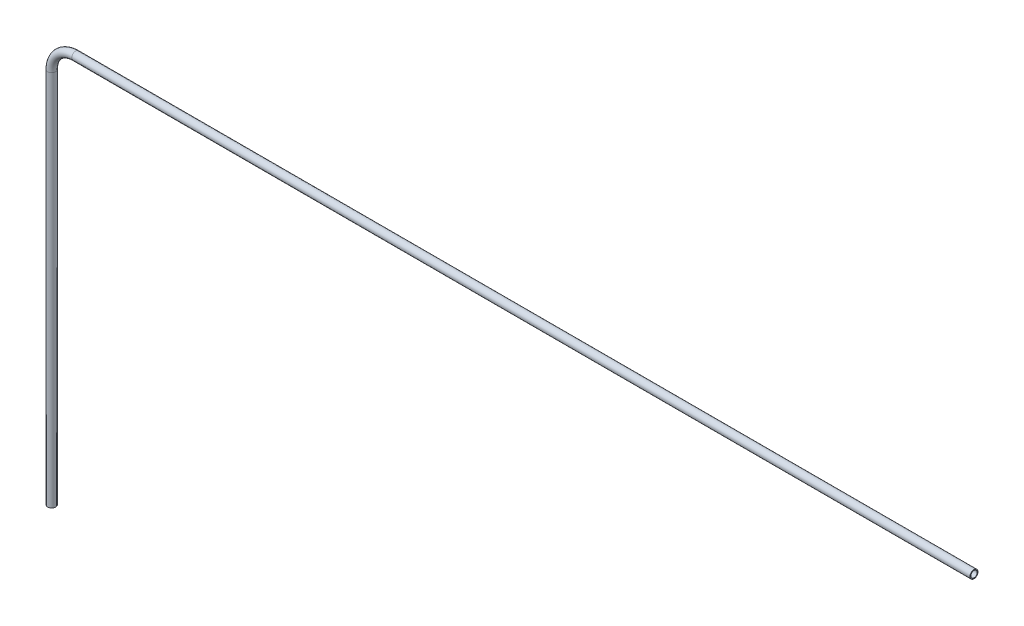
from build123d import *

# Parameters (mm, degrees)
SWEEP_THIN1_PROFILE_R   = 10
SWEEP_THIN1_PROFILE_R_2 = 8


with BuildPart() as part:
    # Sweep-Thin1: sweep along a path in Sketch1
    with BuildLine(Plane.XY) as sweep_thin1_path:
        Line((2300, 0), (60, 0))
        ThreePointArc((60, 0), (17.573593129, -17.573593129), (0, -60))
        Line((0, -60), (0, -1000))
    # Sweep-Thin1 profile (on start of the path) → Sweep-Thin1 (sweep)
    with BuildSketch(Plane(origin=(2300, 0, 0), x_dir=(0, 0, -1), z_dir=(-1, 0, 0))):
        Circle(SWEEP_THIN1_PROFILE_R)
        Circle(SWEEP_THIN1_PROFILE_R_2, mode=Mode.SUBTRACT)
    sweep(path=sweep_thin1_path.line)


solid = part.part
